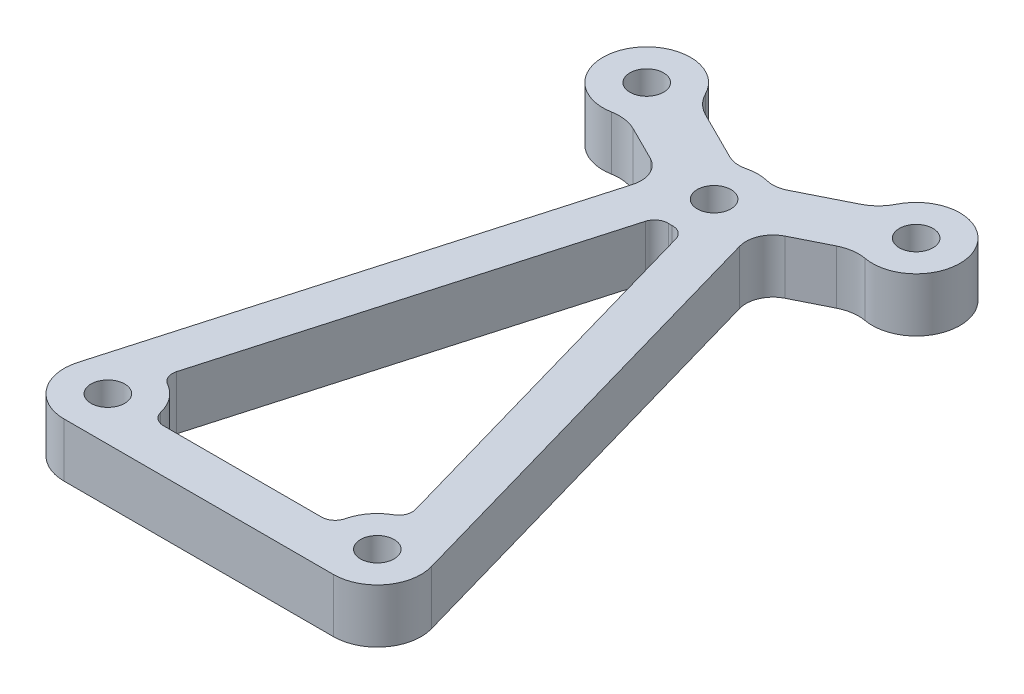
SolidWorks part; units mm, degrees
material "6061 合金"
ref_plane "前视基准面" through (0, 0, 0) normal (0, 0, 1) x (1, 0, 0)
ref_plane "上视基准面" through (0, 0, 0) normal (0, 1, 0) x (1, 0, 0)
ref_plane "右视基准面" through (0, 0, 0) normal (1, 0, 0) x (0, 0, -1)
other "Configuration Table"
sketch "草图1" plane through (0, 0, 0) normal (0, 1, 0) x (1, 0, 0)
  line L0 (0, 0) -> (0, 35) construction
  line L1 (0, 0) -> (10, 0) construction
  line L2 (0, 35) -> (-10, 0) construction
  line L5 (-10, 0) -> (10, 0) construction
  line L8 (10, 0) -> (0, 35) construction
  line L11 (-9.1072, 3.125) -> (-0.8928, 31.875)
  line L12 (-6.75, 0) -> (6.75, 0)
  line L13 (0.8928, 31.875) -> (9.1072, 3.125)
  line L14 (-13.125, 0.8928) -> (-3.125, 35.8928)
  line L15 (3.125, 35.8928) -> (13.125, 0.8928)
  line L16 (-10, -3.25) -> (10, -3.25)
  line L17 (0, 35) -> (10, 40) construction
  line L18 (1.3969, 37.9345) -> (6.8143, 40.6432)
  line L19 (3.1857, 34.3568) -> (8.6031, 37.0655)
  line L20 (-3.1857, 34.3568) -> (-8.6031, 37.0655)
  line L21 (-1.3969, 37.9345) -> (-6.8143, 40.6432)
  circle A0 centre (0, 35) radius 1.25
  circle A1 centre (10, 0) radius 1.25
  circle A2 centre (-10, 0) radius 1.25
  circle A9 centre (0, 35) radius 3.25
  circle A10 centre (-10, 0) radius 3.25
  circle A11 centre (10, 0) radius 3.25
  circle A12 centre (10, 40) radius 1.25
  circle A13 centre (-10, 40) radius 1.25
  circle A14 centre (10, 40) radius 3.25
  circle A15 centre (-10, 40) radius 3.25
  dimension "D1" = 2.5
  dimension "D4" = 40
  dimension "6" = 6.5
  dimension "D2" = 35
  dimension "D3" = 10
  dimension "D5" = 4
extrude "凸台-拉伸1" add sketch "草图1" along normal blind 4 contours A15 A13 | A15 L20 L14 A9 L21 | A10 L11 A9 L20 L14 | A11 L15 L19 A9 L13 | A10 A2 | A11 L12 A10 L16 | A11 A1 | A9 A0 | A9 L14 L20 | A9 L19 L15 | A14 L18 A9 L15 L19 | A14 A12
fillet "圆角1" radius 1 6 edges at (9.1072, 2, -3.125) (6.75, 2, 0) (-6.75, 2, 0) (-9.1072, 2, -3.125) (0.8928, 2, -31.875) (-0.8928, 2, -31.875)
fillet "圆角2" radius 2 4 edges at (-1.3969, 2, -37.9345) (1.3969, 2, -37.9345) (3.5166, 2, -34.5222) (-3.5166, 2, -34.5222)
fillet "圆角3" radius 3 4 edges at (8.6031, 2, -37.0655) (6.8143, 2, -40.6432) (-6.8143, 2, -40.6432) (-8.6031, 2, -37.0655)
